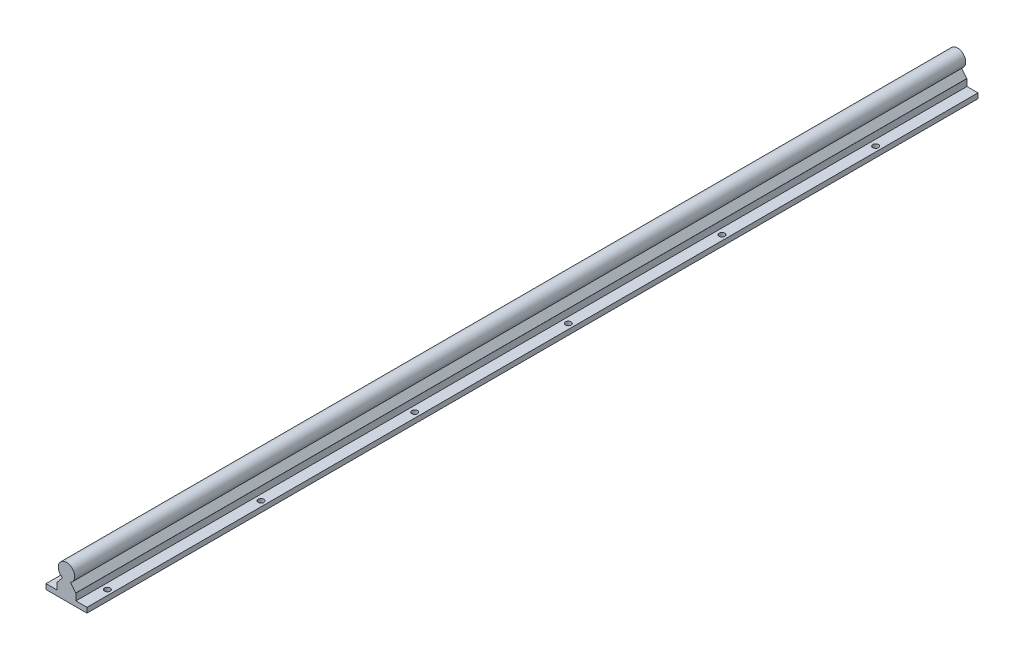
SolidWorks part; units mm, degrees
ref_plane "主视基准图" through (0, 0, 0) normal (0, 0, 1) x (1, 0, 0)
ref_plane "上视基准图" through (0, 0, 0) normal (0, 1, 0) x (1, 0, 0)
ref_plane "右视基准图" through (0, 0, 0) normal (1, 0, 0) x (0, 0, -1)
sketch "草图1" plane through (0, 0, 0) normal (0, 0, 1) x (1, 0, 0)
  line L0 (-9.25, 11.7) -> (-9.25, 5)
  line L1 (-9.25, 5) -> (-20, 5)
  line L2 (-20, 5) -> (-20, 0)
  line L3 (-20, 0) -> (20, 0)
  line L4 (20, 0) -> (20, 5)
  line L5 (20, 5) -> (9.25, 5)
  line L6 (9.25, 5) -> (9.25, 11.7)
  line L7 (9.25, 11.7) -> (9.1185, 11.7)
  line L8 (9.1185, 11.7) -> (4, 17.8)
  line L9 (4, 17.8) -> (3.4871, 17.8)
  line L10 (-3.4871, 17.8) -> (-4, 17.8)
  line L11 (-4, 17.8) -> (-9.1185, 11.7)
  line L12 (-9.1185, 11.7) -> (-9.25, 11.7)
  arc A0 (-3.4871, 17.8) -> (3.4871, 17.8) centre (0, 25) ccw
extrude "凸台-拉伸1" add sketch "草图1" along normal mid plane 870
sketch "草图2" plane through (0, 0, 435) normal (0, 0, 1) x (1, 0, 0)
  arc A0 (3.4871, 17.8) -> (-3.4871, 17.8) centre (0, 25) ccw
  arc A1 (-3.4871, 17.8) -> (3.4871, 17.8) centre (0, 25) ccw
  arc A2 (-3.4871, 17.8) -> (3.4871, 17.8) centre (0, 25) ccw construction
extrude "凸台-拉伸2" add sketch "草图2" against normal up to surface (870 mm away) up to face at (0, 9.8, -435)
hole_wizard "Ø5.5 (5.5) 直径孔1" positions "草图4" profile "草图3" hole size "Ø5.5" standard "Ansi Metric"
sketch "草图4" plane through (0, 5, 0) normal (0, 1, 0) x (1, 0, 0)
  line L0 (0, 435) -> (0, 396.7184) construction
  line L1 (8, 435) -> (-8, 435) construction
  line L4 (20, -435) -> (9.25, -435) construction
  point P0 (15, -410)
  point P2 (-15, -410)
  dimension "D1" = 30
  dimension "D2" = 25
sketch "草图3" plane through (15, 5, 410) normal (1, 0, 0) x (0, 0, 1)
  line L0 (0, 0) -> (0, 17.1977)
  line L1 (0, 17.1977) -> (2.75, 15.61)
  line L2 (2.75, 15.61) -> (2.75, 0)
  line L5 (2.75, 0) -> (0, 0)
  line L10 (0, 17.1977) -> (-2.75, 15.61) construction
  line L11 (0, -6.35) -> (0, 107.95) construction
  dimension "孔直径" = 5.5
  dimension "孔深度" = 15.61
  dimension "导头角度" = 120
pattern_linear "阵列(线性)1" count 6 spacing 150 along (0, 0, -1) of "Ø5.5 (5.5) 直径孔1"
